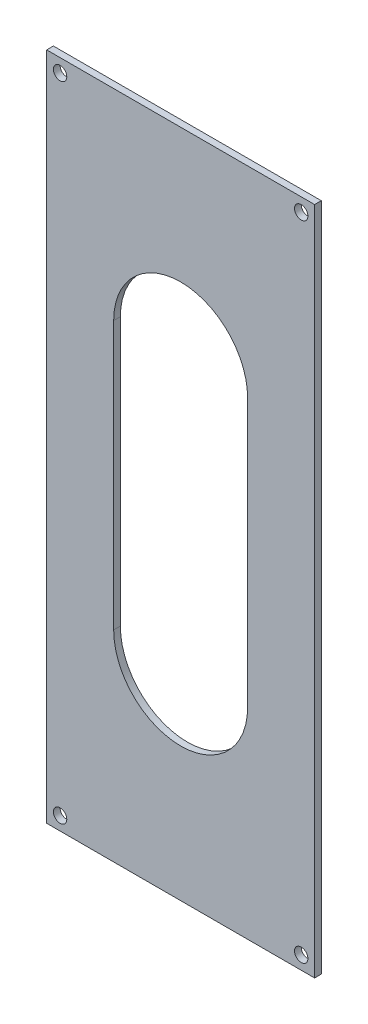
from build123d import *

# Parameters (mm, degrees)
SKETCH1_W           = 400
SKETCH1_H           = 1000
BOSS_EXTRUDE1_DEPTH = 10
SKETCH2_R           = 10
CUT_EXTRUDE1_DEPTH  = 42
CUT_EXTRUDE2_DEPTH  = 20


with BuildPart() as part:
    # Sketch1 → Boss-Extrude1 (new body)
    with BuildSketch(Plane.XY):
        Rectangle(SKETCH1_W, SKETCH1_H)
    extrude(amount=BOSS_EXTRUDE1_DEPTH)

    # Sketch2 → Cut-Extrude1 (cut)
    with BuildSketch(Plane(origin=(0, 0, 0), x_dir=(-1, 0, 0), z_dir=(0, 0, -1))):
        with Locations((-180, 480)):
            Circle(SKETCH2_R)
        with Locations((180, 480)):
            Circle(SKETCH2_R)
        with Locations((180, -480)):
            Circle(SKETCH2_R)
        with Locations((-180, -480)):
            Circle(SKETCH2_R)
    extrude(amount=-CUT_EXTRUDE1_DEPTH, mode=Mode.SUBTRACT)

    # Sketch3 → Cut-Extrude2 (cut)
    with BuildSketch(Plane.XY.offset(10)):
        with BuildLine():
            Line((100, 200), (100, -200))
            ThreePointArc((100, -200), (0, -300), (-100, -200))
            Line((-100, -200), (-100, 200))
            ThreePointArc((-100, 200), (0, 300), (100, 200))
        make_face()
    extrude(amount=-CUT_EXTRUDE2_DEPTH, mode=Mode.SUBTRACT)


solid = part.part
